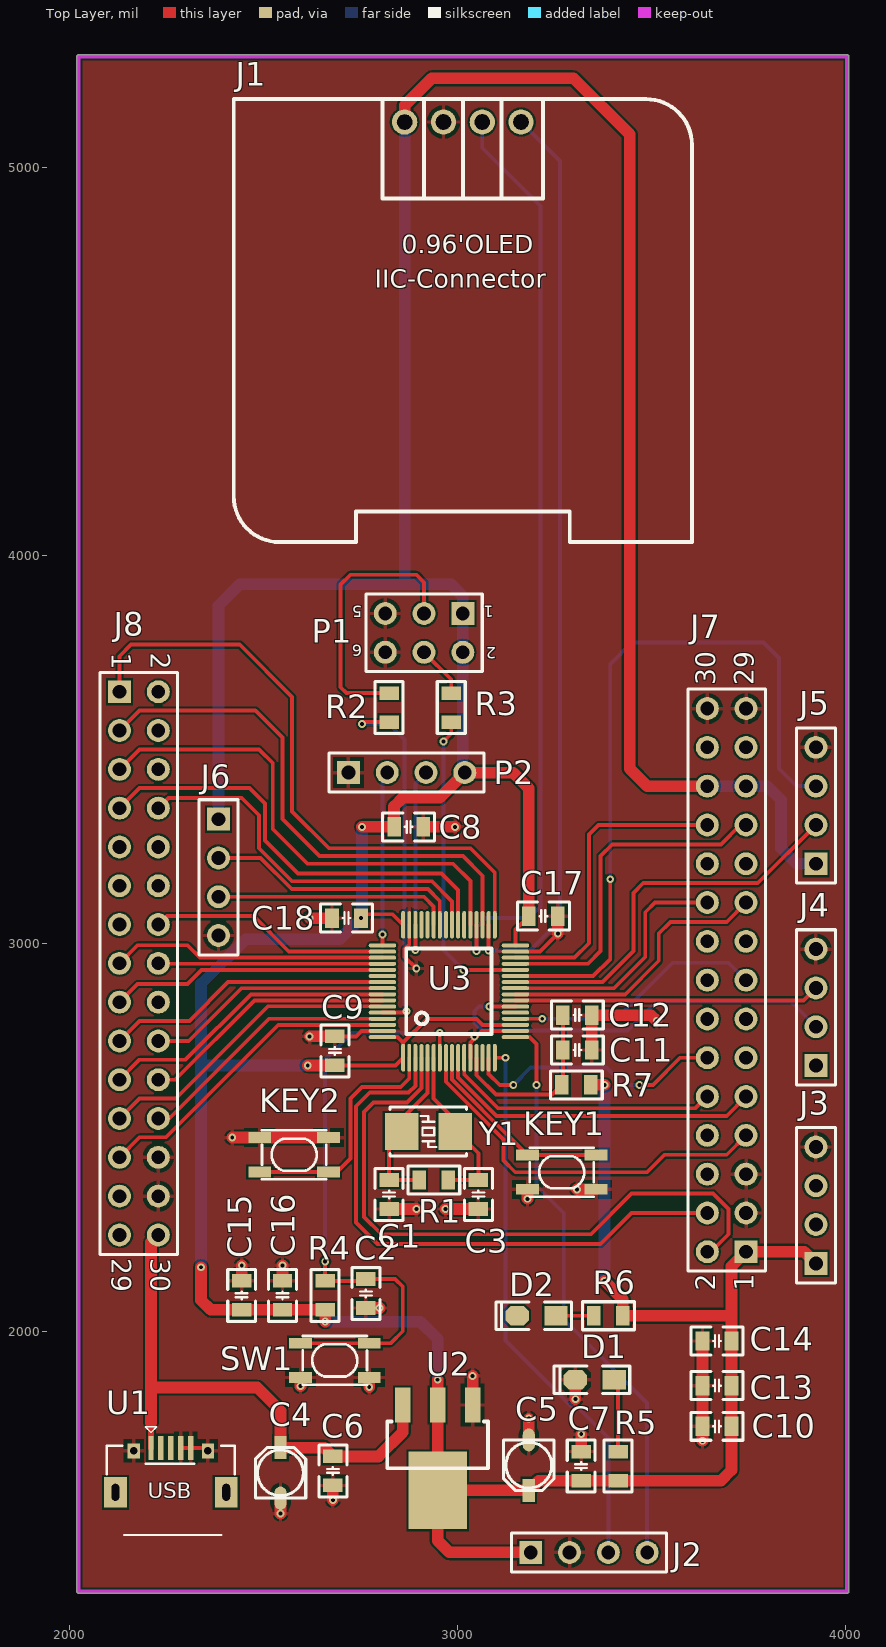
[diagram p0: Top Layer view]
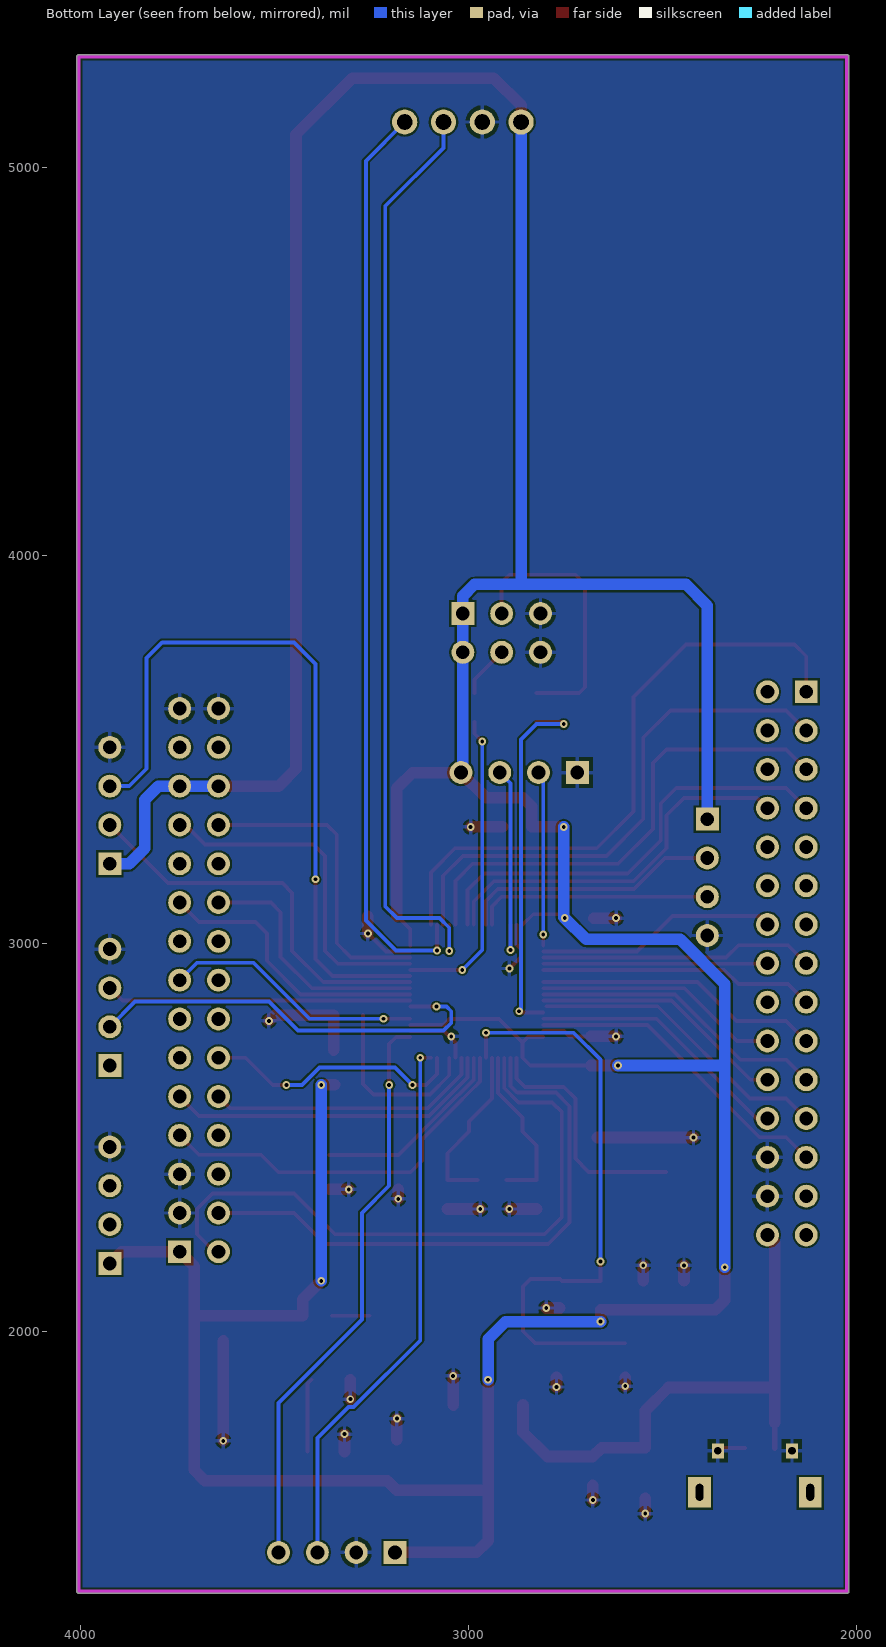
[diagram p1: Bottom Layer view, seen from below]
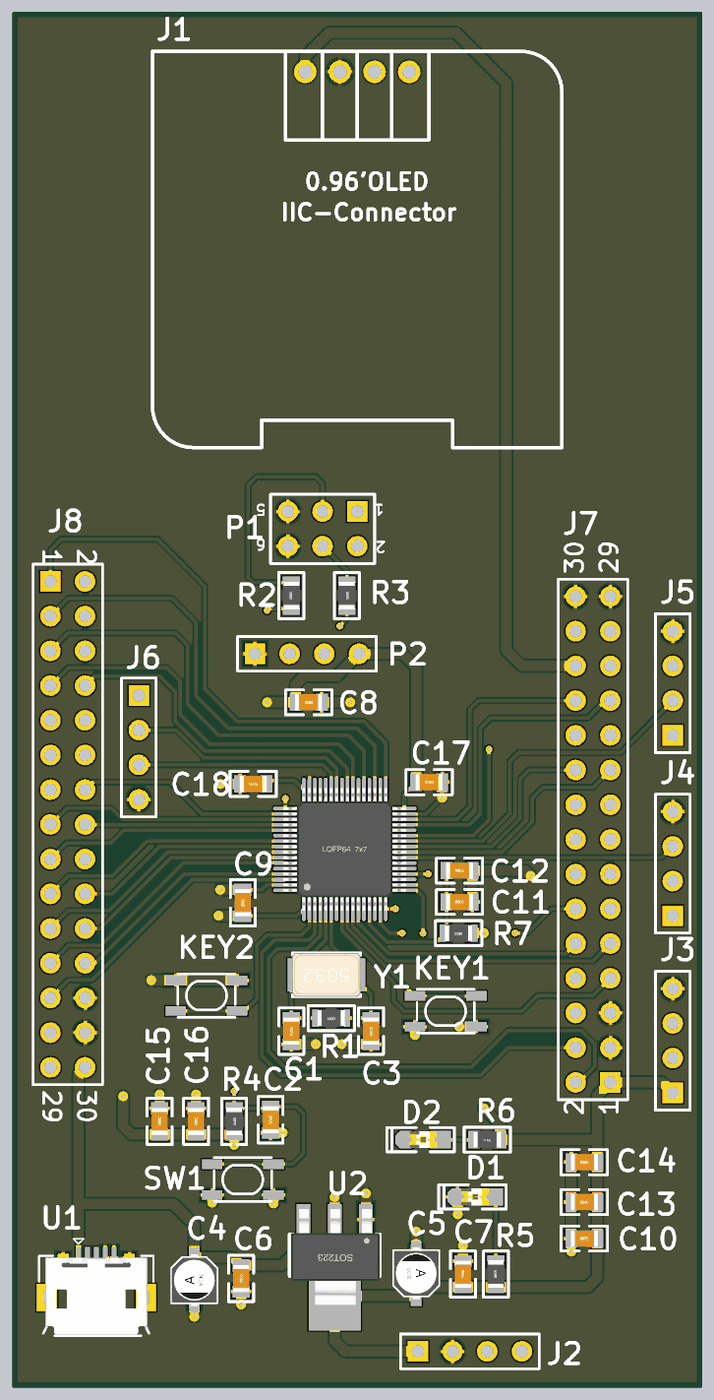
[diagram p2: 3D render of the assembled board from above, using the file's embedded part models]
# Altium PCB MISC62810.PcbDoc
Units mil, origin at the board's own origin, x right, y up, seen from the top; angles counter-clockwise.
Board outline 1990.03 x 3965.03 mil, 2 copper layers (Top Layer, Bottom Layer); 44 components, 73 nets, 239 pads, 49 vias.
Unrouted connection lines stored in the file: 1.

## Layer stack, top to bottom (the 12.6 mil dielectric is the usual default, probably not edited)
Top Solder: solder mask 0.4, Solder Resist, Dk 3.5
Top Layer: signal copper 1.4
Dielectric 1: dielectric 12.6, FR-4, Dk 4.8
Bottom Layer: signal copper 1.4
Bottom Solder: solder mask 0.4, Solder Resist, Dk 3.5

## Board outline
2019.98,1330 ccw(c2025,1330) 2025,1324.98 4005,1324.98 ccw(c4005,1330) 4010.01,1330 4010.01,5285 ccw(c4005,5285) 4005,5290.02 2025,5290.02 ccw(c2025,5285) 2019.98,5285

## Design rules (kind name [scope] priority, off if disabled: settings)
Clearance [All] p1: gap=5
MinimumSolderMaskSliver [All] p1: minsoldermaskwidth=0
PolygonConnect [All] p1: connectstyle=Relief reliefconductorwidth=10 reliefentries=4 polygonreliefangle="90 Angle" airgapwidth=10
RoutingVias [All] p1: holewidth=28 width=50 viastyle="Through Hole" minholewidth=28 minwidth=50 maxholewidth=28 maxwidth=50
SilkToSilkClearance [All] p1: silktosilkclearance=0
SilkToSolderMaskClearance [IsPad] p1: minsilkscreentomaskgap=0 clearancetoexposedcopper=TRUE
SolderMaskExpansion [All] p1: expansion=4
Width [All] p1: maxlimit=30 minlimit=10 preferedwidth=10
27 further rules are at their usual default settings.

## Components (designator, comment, footprint, x,y, rotation, side; value= is the part's Value field where it differs from the comment)
C1 "Cap" "C 0805_L" 2825,2352.6 r90 top
C2 "" "C 0805_L" 2765,2097.4 r90 top
C3 "Cap" "C 0805_L" 3055,2352.6 r90 top
C4 "Cap Pol1" "CM A(3*5.4)" 2545,1635 r90 top
C5 "Cap Pol1" "CM A(3*5.4)" 3185,1655 r270 top
C6 "Cap" "C 0805_L" 2680,1640 r90 top
C7 "Cap" "C 0805_L" 3320,1652.6 r270 top
C8 "Cap" "C 0805_L" 2875,3300 r180 top
C9 "Cap" "C 0805_L" 2685,2722.6 r270 top
C10 "Cap" "C 0805_L" 3670,1755 r0 top
C11 "Cap" "C 0805_L" 3310,2725 r0 top
C12 "Cap" "C 0805_L" 3310,2815 r0 top
C13 "Cap" "C 0805_L" 3670,1860 r180 top
C14 "Cap" "C 0805_L" 3670,1975 r180 top
C15 "Cap" "C 0805_L" 2445,2092.6 r270 top
C16 "Cap" "C 0805_L" 2550,2092.6 r270 top
C17 "Cap" "C 0805_L" 3222.4,3070 r180 top
C18 "Cap" "C 0805_L" 2715,3065 r0 top
D1 "LED0" "LED 0805G" 3355,1875 r180 top
D2 "LED0" "LED 0805G" 3205,2040 r180 top
J1 "OLED" 0.96OLED_4P 3015,4605 r0 top
J2 "SIM900A" HDR1X4 3190,1430 r0 top
J3 "HC-SR04" HDR1X4 3925,2175 r90 top
J4 "HC-SR04" HDR1X4 3925,2685 r90 top
J5 "HC-SR04" HDR1X4 3925,3205 r90 top
J6 "HC-SR04" HDR1X4 2385,3320 r270 top
J7 "HEADER 15X2" HDR2X15 3745,2205 r90 top
J8 "HEADER 15X2" HDR2X15 2130,3648.31 r270 top
KEY1 "SW-PB" "TSW SMD-3*4*2.5" 3270,2410 r180 top
KEY2 "SW-PB" "TSW SMD-3*4*2.5" 2580,2455 r0 top
P1 "Header 3X2" HDR2X3 3015,3850 r180 top
P2 "SWD" HDR1X4 2720,3440 r0 top
R1 "" "R 0805_L" 2940,2390 r180 top
R2 "Res2" "R 0805_L" 2825,3607.6 r90 top
R3 "Res2" "R 0805_L" 2985,3607.6 r270 top
R4 "Res2" "R 0805_L" 2660,2092.6 r270 top
R5 "Res1" "R 0805_L" 3415,1652.6 r90 top
R6 "Res1" "R 0805_L" 3390,2040 r180 top
R7 "Res2" "R 0805_L" 3307.4,2635 r180 top
SW1 "SW-PB" "TSW SMD-3*4*2.5" 2685,1925 r180 top
U1 "USB-Micro" USB-MICRO_B 2211.1,1699.17 r0 top
U2 "AMS1117-3.3" SOT223 2950,1810 r180 top
U3 "STM32F103RCT6" "LQFP64 7x7" 2979.13,2876.35 r0 top
Y1 "8M" "OSC 5032-2P" 2926.1,2515 r180 top

## Footprints (in the part's own frame and the unit in brackets; to place one, negate y for a bottom-side part, rotate by r counter-clockwise, add the part's x,y. Pads: shape width x height; smd on the part's side, far side on the other; paste and mask are expansions set on the pad)
0.96OLED_4P [mm]
  round 1.65 hole 1 slot 1.005 at 0 deg paste+0 mask+0.051: 1(-3.811,12.997) 2(-1.271,13) 3(1.269,13) 4(3.809,13)
  silkscreen extent -15,-14.5 15,14.5
"C 0805_L" [mil] "无极性贴片电容"
  rect 35x50 smd: 1(-37.4,0) 2(37.4,0)
  silkscreen extent -67,-36 67,36, body extent -39,-24 39,24, height 20
"CM A(3*5.4)" [mm] "贴片电解电容，直径3mm，高5.4mm"
  rect 1.5x0.8 smd: 1(1.651,0)
  oval 1.5x0.8 smd: 2(-1.65,0)
  silkscreen extent -1.65,-1.65 1.65,1.65, body extent -1.9,-1.65 1.9,1.65, height 5.4
HDR1X4 [mm] "Connector; Header; 4 Position"
  rect 1.5x1.5 hole 0.9: 1(0,0)
  round 1.5 hole 0.9: 2(2.54,0) 3(5.08,0) 4(7.62,0)
  silkscreen extent -1.27,-1.27 8.89,1.27
HDR2X3 [mm]
  rect 1.5x1.5 hole 0.9: 1(0,0)
  round 1.5 hole 0.9: 2(0,2.54) 3(2.54,0) 4(2.54,2.54) 5(5.08,0) 6(5.08,2.54)
  silkscreen extent -1.27,-1.27 6.35,3.81
HDR2X15 [mm] "Connector; Header; 15x2 Position"
  rect 1.5x1.5 hole 0.9: 1(0,0)
  round 1.5 hole 0.9: 2(0,2.54) 3(2.54,0) 4(2.54,2.54) 5(5.08,0) 6(5.08,2.54) 7(7.62,0) 8(7.62,2.54) 9(10.16,0) 10(10.16,2.54) 11(12.7,0) 12(12.7,2.54) 13(15.24,0) 14(15.24,2.54) 15(17.78,0) 16(17.78,2.54) 17(20.32,0) 18(20.32,2.54) 19(22.86,0) 20(22.86,2.54) 21(25.4,0) 22(25.4,2.54) 23(27.94,0) 24(27.94,2.54) 25(30.48,0) 26(30.48,2.54) 27(33.02,0) 28(33.02,2.54) 29(35.56,0) 30(35.56,2.54)
  silkscreen extent -1.27,-1.27 36.83,3.81
"LED 0805G" [mil] "绿色0805LED"
  rect 60x50 smd: 1(-50,0)
  oct 60x50 smd: 2(50,0)
  silkscreen extent -90,-35 105,35, body extent -39,-25 39,25, height 32
"LQFP64 7x7" [mm]
  oval 0.26x1.8 smd: 1(-3,-4.352) 2(-2.6,-4.352) 3(-2.2,-4.352) 4(-1.8,-4.352) 5(-1.4,-4.352) 6(-1,-4.352) 7(-0.6,-4.352) 8(-0.2,-4.352) 9(0.2,-4.352) 10(0.6,-4.352) 11(1,-4.352) 12(1.4,-4.352) 13(1.8,-4.352) 14(2.2,-4.352) 15(2.6,-4.352) 16(3,-4.352) 33(3,4.352) 34(2.6,4.352) 35(2.2,4.352) 36(1.8,4.352) 37(1.4,4.352) 38(1,4.352) 39(0.6,4.352) 40(0.2,4.352) 41(-0.2,4.352) 42(-0.6,4.352) 43(-1,4.352) 44(-1.4,4.352) 45(-1.8,4.352) 46(-2.2,4.352) 47(-2.6,4.352) 48(-3,4.352)
  oval 1.8x0.26 smd: 17(4.352,-3) 18(4.352,-2.6) 19(4.352,-2.2) 20(4.352,-1.8) 21(4.352,-1.4) 22(4.352,-1) 23(4.352,-0.6) 24(4.352,-0.2) 25(4.352,0.2) 26(4.352,0.6) 27(4.352,1) 28(4.352,1.4) 29(4.352,1.8) 30(4.352,2.2) 31(4.352,2.6) 32(4.352,3) 49(-4.352,3) 50(-4.352,2.6) 51(-4.352,2.2) 52(-4.352,1.8) 53(-4.352,1.4) 54(-4.352,1) 55(-4.352,0.6) 56(-4.352,0.2) 57(-4.352,-0.2) 58(-4.352,-0.6) 59(-4.352,-1) 60(-4.352,-1.4) 61(-4.352,-1.8) 62(-4.352,-2.2) 63(-4.352,-2.6) 64(-4.352,-3)
  silkscreen extent -2.79,-2.79 2.79,2.79, body extent -4.51,-4.5 4.5,4.5, height 1.45
"OSC 5032-2P" [mm] "5mm*3.2mm*0.8mm(长*宽*高)"
  rect 2.2x2.4 smd: 1(-1.75,0) 2(1.75,0)
  silkscreen extent -2.5,-1.6 2.5,1.6, body extent -2.5,-1.6 2.5,1.6, height 0.86
"R 0805_L" [mil] "1/8W贴片电阻"
  rect 35x50 smd: 1(-37.4,0) 2(37.4,0)
  silkscreen extent -67,-36 67,36, body extent -39,-25 39,25, height 20
SOT223 [mil]
  rect 40x90 smd: 1(-90,0) 2(0,0) 3(90,0)
  rect 150x200 smd: 2(0,220)
  silkscreen extent -130,43 130,163, body extent -130,-30 126,246, height 65
"TSW SMD-3*4*2.5" [mm] "3*4*2.5mm"
  rect 1.5x0.7 smd: 1(-2.25,1.125) 1(2.25,1.125) 2(-2.25,-1.125) 2(2.25,-1.125)
  silkscreen extent -2.1,-1.6 2.1,1.6
USB-MICRO_B [mm]
  rect 1.5x2 hole 0.5 slot 1.1 at 90 deg: 0(-2.325,-2.9) 0(4.925,-2.9)
  rect 0.35x1.6 smd: 1(0,0) 2(0.65,0) 3(1.3,0) 4(1.95,0) 5(2.6,0)
  rect 0.8x1 hole 0.5: 5(-1.125,-0.19) 5(3.725,-0.19)
  silkscreen extent -2.89,-5.69 5.49,1.4, body extent -2.7,-5.6 5.3,0, height 2.8

## Part data
C1 C3 C6 C7 C8 C9 C10 C11 C12 C13 C14 C15 C16 C17 C18: "Capacitor"
C2: library part Cap, "Capacitor"
C4 C5: "Polarized Capacitor (Radial)"
D1 D2: "Typical INFRARED GaAs LED"
J1 J3 J4 J5 J6 P2: library part "Header 4", "Header, 4-Pin"
J2 U1 U2 U3: library part Component_1
J7 J8: library part "Header 15X2", "Header, 15-Pin, Dual row"
KEY1 KEY2 SW1: "Switch"
P1: "Header, 3-Pin, Dual row"
R1: library part Res2, "Resistor"
R2 R3 R4 R5 R6 R7: "Resistor"
Y1: library part XTAL, "Crystal Oscillator"

## Via types
v1: diameter 20, hole 10, Top Layer to Bottom Layer, 49 vias

## Nets (pads, with @x,y where several pads share a name; then routed paths per layer and width w, separated by ;. In a path a pad name is that pad's centre, name@x,y a point inside that pad or via, vN(x,y) a via of type N, cw(c..) or ccw(c..) an arc to the next point about the centre after c; other vN are vias at no path point)
3V3: C5.1 C7.2 C8.2 C9.2 C10.2 C13.1 C14.1 C15.2 C16.2 C17.2 C18.2 J1.1 J2.1 J3.1 J4.1 J5.1 J6.1 J7.1 J7.25 J7.26 P1.1 P1.2 P2.4 R4.2 R5.1 R6.1 R7.1 U2.2 U3.1 U3.19 U3.32 U3.48 U3.64 | length 13352.9
  Top Layer w10: C9.2 2841.22,2685.2 U3.1 2861.02,2743.98 ; v1(2752.4,3065) 2762.4,3075 2833.73,3075 U3.48 ; U3.64 2846.76,2758.24 2861.02,2743.98 ; U3.19 3065.26,2789.74 3050,2805 2922.05,2805 2861.02,2743.98 ; U3.32 3150.49,3035.49 C17.2
  Top Layer w30: v1(2340,2165) 2340,2080 2364.8,2055.2 C15.2 C16.2 R4.2 v1(2660,2025) ; v1(2615.2,2685.2) C9.2 ; v1(2755,3300) C8.2 2837.6,3352.6 2860,3375 2955,3375 P2.4 3145,3440 3185,3400 C17.2 ; J1.1 2864.95,5159.95 2935,5230 3300,5230 3445,5085 3445,3450 3490,3405 J7.26 ; v1(2950,1875) 2950,1810 U2.2@2950,1590 ; J2.1 2980,1430 2950,1460 U2.2@2950,1590 ; R7.1 v1(3380,2635) ; v1(3380,2130) 3427.4,2082.6 R6.1 3707.4,2040 ; J3.1 3895,2205 J7.1 3707.4,2167.4 3707.4,2040 ; U2.2@2950,1590 C5.1 3210.2,1615.2 C7.2 R5.1 3680.2,1615.2 3707.4,1642.4 C10.2 C14.1 3707.4,2040
  Bottom Layer w30: v1(2340,2165) 2340,2680 ; J6.1 2385,3870 2440,3925 2860,3925 ; v1(2615.2,2685.2) 2345.2,2685.2 2340,2680 ; v1(2660,2025) 2905,2025 2950,1980 v1(2950,1875) ; v1(2755,3300) 2755,3067.6 v1(2752.4,3065) 2697.4,3010 2455,3010 2340,2895 2340,2680 ; J1.1 2864.95,3929.95 2860,3925 ; P2.4 3015,3445 P1.2 P1.1 3015,3895 2985,3925 2860,3925 ; v1(3380,2130) v1(3380,2635) ; J7.26 J7.25 3800,3405 3835,3370 3835,3245 3875,3205 J5.1
5V: C4.1 C6.2 J8.30 U1.1 U2.3 | length 1431
  Top Layer w15: U1.1 2211.1,1763.9
  Top Layer w30: 2211.1,1763.9 2211.1,1855 ; J8.30 2211.1,2229.41 2211.1,1855 ; U2.3 2860,1740 2797.4,1677.4 C6.2 2657.4,1700 C4.1 2545,1795 2485,1855 2211.1,1855
BOOT0: R2.1 U3.60 | length 972.1
  Top Layer w10: v1(2755,3565) 2760.2,3570.2 R2.1 ; U3.60 2873.76,2821.24 v1(2870,2825)
  Bottom Layer w10: v1(2755,3565) 2825,3565 2865,3525 2865,2830 v1(2870,2825)
BOOT1: R3.2 U3.28 | length 802.3
  Top Layer w10: v1(2965,3520) 2985,3540 R3.2 ; v1(3016.47,2931.47) U3.28
  Bottom Layer w10: v1(2965,3520) 2965,2982.94 v1(3016.47,2931.47)
ECHO1: J3.3
ECHO2: J4.3 U3.23 | length 787.9
  Top Layer w10: U3.23 3892.73,2852.73 J4.3
ECHO3: J5.3 U3.27 | length 1895.8
  Top Layer w10: U3.27 3350.72,2915.72 3395,2960 v1(3395,3165)
  Bottom Layer w10: v1(3395,3165) 3395,3720 3450,3775 3790,3775 3830,3735 3830,3450 3875,3405 J5.3
ECHO4: J6.3 U3.43 | length 612.5
  Top Layer w10: J6.3 2915,3120 2939.76,3095.24 U3.43
GND: C1.1 C2.1 C3.1 C4.2 C5.2 C6.1 C7.1 C8.1 C9.1 C10.1 C11.2 C12.2 C13.2 C14.2 C15.1 C16.1 C17.1 C18.1 D1.2 J1.2 J2.2 J3.4 J4.4 J5.4 J6.4 J7.3 J7.5 J7.29 J7.30 J8.26 J8.28 KEY1.1 KEY2.1 P1.5 P1.6 P2.1 SW1.1 U1.4 U1.5 U2.1 U3.12 U3.18 U3.31 U3.47 U3.63 | length 2339.7
  Top Layer w10: U1.4 2313.46,1699.17 2350.28,1699.17 U1.5@2357.76,1691.69 ; C9.1 2740,2760 2753.99,2773.99 U3.63 ; U3.47 2876.77,2996.77 2865,2985 2865,2965 v1(2895,2935) ; U3.12 3034.25,2744.25 3063.99,2773.99 U3.18 ; U3.31 3213.32,2978.72 v1(3259.8,3025.2)
  Top Layer w30: v1(2420.71,2499.29) 2491.42,2499.29 KEY2.1@2668.58,2499.29 ; C15.1 v1(2445,2170) ; v1(2545,1530) C4.2 ; C16.1 v1(2550,2170) ; v1(2596.42,1858.58) SW1.1@2596.42,1880.71 ; v1(2620,2760) C9.1 ; v1(2620,3065) C18.1 ; v1(2680,1565) C6.1 ; C2.1 v1(2800,2060) ; v1(2773.58,1856.42) SW1.1@2773.58,1880.71 ; C1.1 v1(2895.2,2315.2) ; C8.1 v1(2995,3300) ; v1(2970.2,2315.2) C3.1 ; U2.1 v1(3040,1885) ; v1(3181.42,2341.42) KEY1.1@3181.42,2365.71 ; C5.2 v1(3185,1775) ; v1(3259.8,3025.2) C17.1 ; v1(3305,1825) D1.2 ; v1(3309.29,2365.71) KEY1.1@3358.58,2365.71 ; C7.1 v1(3320,1735) ; C11.2 C12.2 3500,2815 v1(3515,2800) ; v1(3632.6,1717.6) C10.1 C14.2
  other v1: 3045,2760
KEY0: KEY1.2 U3.9 | length 508.5
  Top Layer w10: U3.9 2987.01,2648.7 2987.76,2647.95 2987.95,2647.95 3063.31,2572.6 3063.31,2572.4 3181.42,2454.29 KEY1.2@3358.58,2454.29
KEY1: KEY2.2 U3.2 | length 629.2
  Top Layer w10: KEY2.2@2491.42,2410.71 2668.58,2410.71 2690.71,2410.71 2725,2445 2725,2600 2755,2630 2855,2630 2876.77,2651.77 U3.2
LED0: U3.41
NetC11_1: C11.1 C12.1 R7.2 U3.13 | length 477.1
  Top Layer w10: U3.13 3050,2660 3100,2610 3245,2610 R7.2 3272.6,2637.6 C11.1 C12.1
NetD1_1: D1.1 R5.2 | length 189.1
  Top Layer w10: D1.1 3415,1865 R5.2
NetD2_1: D2.1 R6.2 | length 97.6
  Top Layer w10: D2.1 R6.2
NetP1_3: P1.3 R2.2 | length 709.9
  Top Layer w10: R2.2 2715,3645 2700,3660 2700,3925 2725,3950 2895,3950 2915,3930 P1.3
NetP1_4: P1.4 R3.1 | length 134
  Top Layer w10: P1.4 2985,3680 R3.1
"OSC _IN2": C1.2 R1.2 U3.5 Y1.2 | length 433.6
  Top Layer w10: R1.2 C1.2 2825,2478.9 2861.1,2515 2861.1,2551.1 2924.02,2614.02 U3.5
OSC_OUT2: C3.2 R1.1 U3.6 Y1.1 | length 440.3
  Top Layer w10: U3.6 2939.76,2600.24 2998.9,2541.1 2998.9,2515 3055,2458.9 C3.2 R1.1
PA0: U3.14
PA1: J7.12 U3.15 | length 683.1
  Top Layer w10: U3.15 3081.5,2663.5 3110,2635 v1(3145,2635) ; v1(3470,2635) 3505,2635 3575,2705 J7.12
  Bottom Layer w10: v1(3145,2635) 3190,2680 3385,2680 3430,2635 v1(3470,2635)
PA4: J7.15 U3.20 | length 673
  Top Layer w10: U3.20 v1(3219.51,2805.49)
  Bottom Layer w10: v1(3219.51,2805.49) 3410.49,2805.49 3555,2950 3700,2950 J7.15
PA5: U3.21
PA6: J7.17
PA8: D2.2
PA11: J8.27
PA12: J8.29
PA13: J8.12
PA14: J8.13
PA15: J8.14 U3.50 | length 624.6
  Top Layer w10: J8.14 2251.69,3070 2475,3070 2566.28,2978.72 U3.50
PB0: J7.21
PB1: J7.22
PB3: J8.19 U3.55 | length 740.6
  Top Layer w10: J8.19 2181.69,2800 2310,2800 2409.98,2899.98 U3.55
PB4: J8.20 U3.56 | length 634.1
  Top Layer w10: J8.20 2308.31,2748.31 2444.23,2884.23 U3.56
PB5: J8.21 U3.57 | length 769
  Top Layer w10: J8.21 2181.69,2700 2300,2700 2468.48,2868.48 U3.57
PB6: J8.22 U3.58 | length 662.5
  Top Layer w10: J8.22 2273.31,2648.31 2477.73,2852.73 U3.58
PB7: J8.23 U3.59 | length 789.8
  Top Layer w10: J8.23 2181.69,2600 2275,2600 2512.61,2837.61 U3.59@2800,2837.61
PB8: J8.24 U3.61 | length 684.3
  Top Layer w10: J8.24 2258.31,2548.31 2515.49,2805.49 U3.61
PB9: J8.25 U3.62 | length 819.2
  Top Layer w10: J8.25 2181.69,2500 2250,2500 2539.11,2789.11 2807.15,2789.11 U3.62
PB10: J7.23 U3.29 | length 886.2
  Top Layer w10: U3.29 3337.22,2947.22 3370,2980 3370,3225 3400,3255 3680,3255 3730,3305 J7.23
PB11: J7.24 U3.30 | length 800.2
  Top Layer w10: U3.30 3302.97,2962.97 3340,3000 3340,3280 3365,3305 J7.24
PB12: J8.1 U3.33 | length 1622.5
  Top Layer w10: J8.1 2130,3740 2160,3770 2440,3770 2575,3635 2575,3340 2670,3245 3035,3245 3097.24,3182.76 U3.33
PB14: J8.3 U3.35 | length 1383.1
  Top Layer w10: J8.3 2181.69,3600 2480,3600 2550,3530 2550,3320 2645,3225 3015,3225 3065.75,3174.25 U3.35
PC0: J7.7 U3.8 | length 1003.5
  Top Layer w10: U3.8 2971.26,2643.43 2972.01,2642.69 2972.01,2642.49 2981.54,2632.95 2981.74,2632.95 3048.31,2566.39 3048.31,2566.19 3120,2494.5 3120,2440 3150,2410 3490,2410 3535,2455 3695,2455 J7.7
PC2: J7.9 U3.10 | length 854.7
  Top Layer w10: U3.10 3002.76,2654.36 3102.12,2555 3695,2555 J7.9
PC3: J7.10 U3.11 | length 718.3
  Top Layer w10: U3.11 3018.5,2661.5 3105,2575 3615,2575 J7.10
PC4: J7.19 U3.24 | length 733.5
  Top Layer w10: U3.24 3433.48,2868.48 3520,2955 3520,3025 3550,3055 3695,3055 J7.19
PC5: J7.20 U3.25 | length 653.3
  Top Layer w10: U3.25 3404.23,2884.23 3485,2965 3485,3080 3510,3105 J7.20
PC6: J8.5 U3.37 | length 1278.8
  Top Layer w10: J8.5 2181.69,3500 2490,3500 2525,3465 2525,3295 2615,3205 2990,3205 3034.25,3160.75 U3.37
PC7: U3.38
PC8: J8.7 U3.39 | length 1148.2
  Top Layer w10: J8.7 2181.69,3400 2465,3400 2505,3360 2505,3265 2590,3180 2960,3180 3002.76,3137.24 U3.39
PC9: J8.8 U3.40 | length 988.7
  Top Layer w10: J8.8 2256.69,3375 2445,3375 2490,3330 2490,3245 2575,3160 2935,3160 2987.01,3107.99 U3.40
PC10: J8.15 U3.51 | length 710.4
  Top Layer w10: J8.15 2176.69,2995 2305,2995 2337.03,2962.97 U3.51
PC11: J8.16 U3.52 | length 578.2
  Top Layer w10: J8.16 2231.09,2947.22 U3.52
PC12: J8.17 U3.53 | length 712.2
  Top Layer w10: J8.17 2176.69,2895 2305,2895 2341.47,2931.47 U3.53
PC14: J7.4 U3.3 | length 1507.7
  Top Layer w10: U3.3 2892.52,2632.52 2875,2615 2775,2615 2740,2580 2740,2280 2795,2225 3370,2225 3450,2305 J7.4
PC15: J7.2 U3.4 | length 1679.3
  Top Layer w10: U3.4 2908.27,2627.05 2871.21,2590 2785,2590 2760,2565 2760,2295 2805,2250 3345,2250 3450,2355 3660,2355 3700,2315 3700,2250 3655,2205 J7.2
PD2: U3.54
RESET: C2.2 R4.1 SW1.2 U3.7 | length 1560.3
  Top Layer w10: SW1.2@2596.42,1969.29 2773.58,1969.29 2829.29,1969.29 2860,2000 2860,2115 2840.2,2134.8 C2.2 2760.2,2130 R4.1 v1(2660,2180) ; U3.7 v1(2955.51,2769.49)
  Bottom Layer w10: v1(2660,2180) 2660,2700 2729.49,2769.49 v1(2955.51,2769.49)
SCL: J1.4 U3.34 | length 2381.3
  Top Layer w10: v1(3081.5,2981.5) U3.34
  Bottom Layer w10: v1(3081.5,2981.5) 3187.82,2981.5 3265,3058.68 3265,5016.75 J1.4
SDI: J1.3 U3.36 | length 2399.4
  Top Layer w10: v1(3050,2980) U3.36
  Bottom Layer w10: v1(3050,2980) 3050,3040 3075,3065 3185,3065 3215,3095 3215,4900 3064.95,5050.05 J1.3
SWDCLK: P2.2 U3.49 | length 450.6
  Top Layer w10: U3.49 v1(2807.78,3022.78)
  Bottom Layer w10: v1(2807.78,3022.78) 2807.78,3427.78 P2.2
SWDIO: P2.3 U3.46 | length 534.1
  Top Layer w10: v1(2892.52,2982.52) U3.46
  Bottom Layer w10: v1(2892.52,2982.52) 2892.52,3412.52 P2.3
TRIG1: J3.2
TRIG2: J4.2 U3.22 | length 1086.7
  Top Layer w10: v1(3083.02,2836.98) U3.22
  Bottom Layer w10: v1(3083.02,2836.98) 3056.98,2836.98 3045,2825 3045,2795 3065,2775 3440,2775 3515,2850 3860,2850 J4.2
TRIG3: J5.2 U3.26 | length 1030.1
  Top Layer w10: U3.26 3374.98,2899.98 3455,2980 3455,3130 3480,3155 3775,3155 J5.2
TRIG4: J6.2 U3.42 | length 678.1
  Top Layer w10: J6.2 2493.79,3220 2573.79,3140 2925,3140 2955.51,3109.49 U3.42
USART2_RX: J2.4 U3.17 | length 1490.1
  Top Layer w10: U3.17 3186.76,2758.24 3205,2740 v1(3205,2635)
  Bottom Layer w10: v1(3205,2635) 3205,2375 3275,2305 3275,2030 3490,1815 J2.4
USART2_TX: J2.3 U3.16 | length 1420.3
  Top Layer w10: U3.16 v1(3125,2705)
  Bottom Layer w10: v1(3125,2705) 3125,1976.72 3296.72,1805 3310,1805 3390,1725 J2.3
"USB D+": U3.45
"USB D-": U3.44
USB_D+: U1.3
USB_D-: U1.2
pads on no net: J7.6 J7.8 J7.11 J7.13 J7.14 J7.16 J7.18 J7.27 J7.28 J8.2 J8.4 J8.6 J8.9 J8.10 J8.11 J8.18 U1.0

## Polygon pours and split planes (outlines as drawn)
GND on Bottom Layer "D" (solid, remove dead copper, pour order 0): 1810,5335 1820,5345 4225,5345 4225,1130 4220,1125 4125,1220 1795,1220
GND on Top Layer "D" (solid, remove dead copper, pour order 2): 1660,5460 4575,5460 4715,5320 4145,4750 4145,1260 2125,1260 1940,1075

## Keep-outs
Keep-Out Layer:
  lines w10: 2025,1450 2025,4050 2025,5285 3905,5285 4005,5285 4005,1330 2245,1330 2050,1330 2025,1330 2025,1460